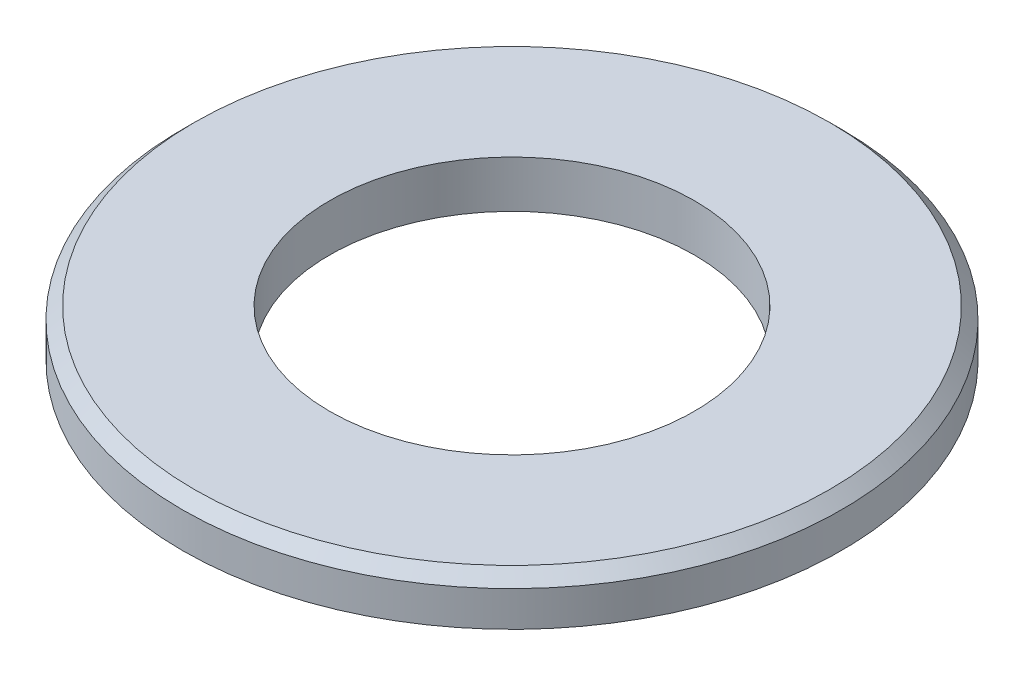
SolidWorks part; units mm, degrees
material "钢"
ref_plane "基准面1" through (0, 0, 0) normal (0, 0, 1) x (1, 0, 0)
ref_plane "基准面2" through (0, 0, 0) normal (0, 1, 0) x (1, 0, 0)
ref_plane "基准面3" through (0, 0, 0) normal (1, 0, 0) x (0, 0, -1)
sketch "尺寸草图" plane through (0, 0, 0) normal (0, 0, 1) x (1, 0, 0)
  line L0 (0, 0) -> (9.1, 0)
  point P3 (4, 0)
  point P4 (56, 0)
  point P5 (31, 0)
sketch "草图1" plane through (0, 0, 0) normal (0, 0, 1) x (1, 0, 0)
  line L0 (0, 0) -> (0, 52.7318) construction
  line L1 (-27, 12.6445) -> (-28, 11.6445)
  line L2 (-15.5, 8.6445) -> (-28, 8.6445)
  line L3 (-15.5, 8.6445) -> (-15.5, 12.6445)
  line L4 (-15.5, 12.6445) -> (-27, 12.6445)
  line L5 (-28, 8.6445) -> (-28, 11.6445)
  point P4 (-28, 12.6445)
revolve "基体-旋转" add sketch "草图1" angle 360 about L0
equation "\"h@草图1\" = \"h@尺寸草图\""
equation "\"D1@草图1\" = \"d1@尺寸草图\" / 2"
equation "\"D2@草图1\" = \"d2@尺寸草图\" / 2"
equation "\"D5@草图1\" = \"h@草图1\" *0.25"
